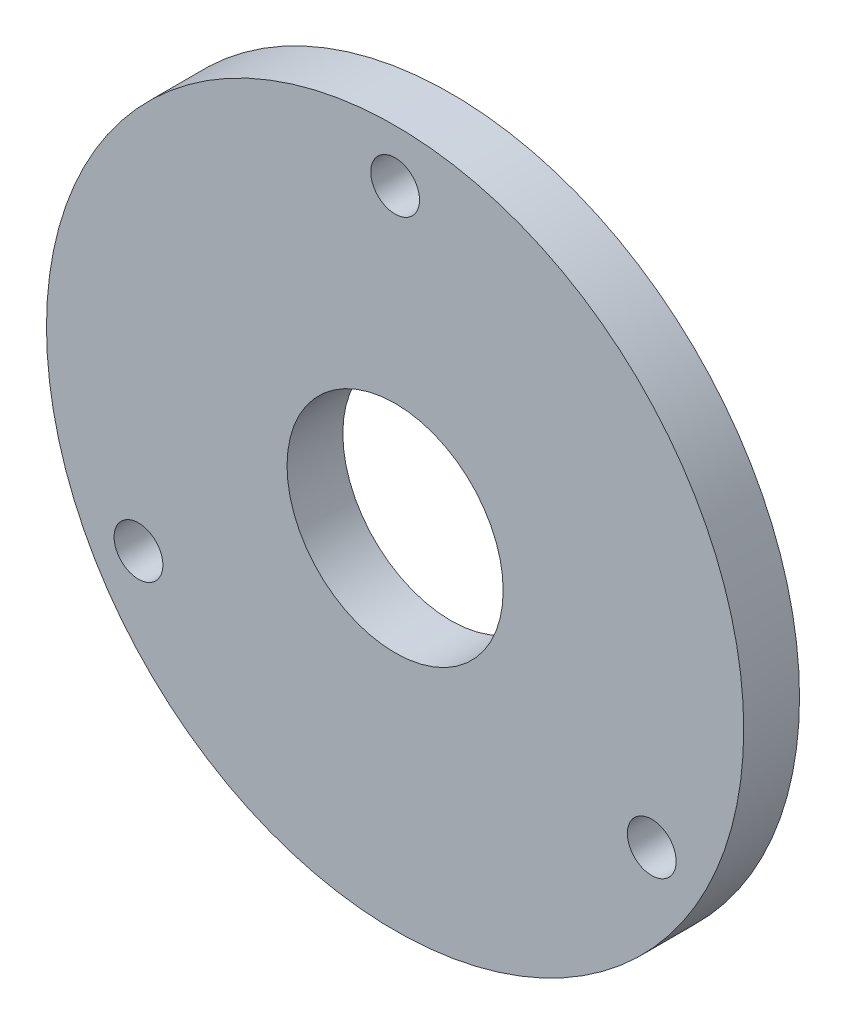
from build123d import *

# Parameters (mm, degrees)
SKETCH1_R           = 50
SKETCH1_R_2         = 3.5
SKETCH1_R_3         = 15.5
BOSS_EXTRUDE1_DEPTH = 8


with BuildPart() as part:
    # Sketch1 → Boss-Extrude1 (new body)
    with BuildSketch(Plane.XY):
        Circle(SKETCH1_R)
        with Locations((0, 42.5)):
            Circle(SKETCH1_R_2, mode=Mode.SUBTRACT)
        with Locations((-36.806079661, -21.25)):
            Circle(SKETCH1_R_2, mode=Mode.SUBTRACT)
        with Locations((36.806079661, -21.25)):
            Circle(SKETCH1_R_2, mode=Mode.SUBTRACT)
        Circle(SKETCH1_R_3, mode=Mode.SUBTRACT)
    extrude(amount=BOSS_EXTRUDE1_DEPTH)


solid = part.part
